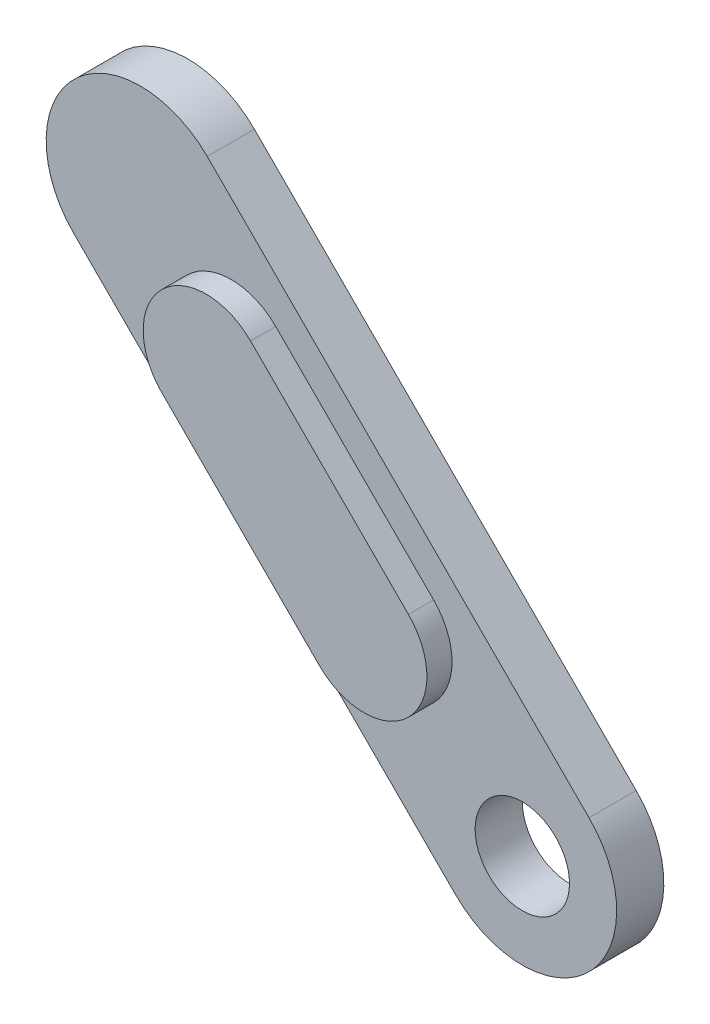
SolidWorks part; units mm, degrees
ref_plane "Front Plane" through (0, 0, 0) normal (0, 0, 1) x (1, 0, 0)
ref_plane "Top Plane" through (0, 0, 0) normal (0, 1, 0) x (1, 0, 0)
ref_plane "Right Plane" through (0, 0, 0) normal (1, 0, 0) x (0, 0, -1)
sketch "Sketch2" plane through (0, 0, 0) normal (0, 0, 1) x (1, 0, 0)
  line L0 (5.5786, 37.7618) -> (-6.5599, 49.9003) construction
  line L1 (7.6999, 39.8831) -> (-4.4386, 52.0216)
  line L2 (3.4572, 35.6405) -> (-8.6812, 47.779)
  arc A0 (3.4572, 35.6405) -> (7.6999, 39.8831) centre (5.5786, 37.7618) ccw
  arc A1 (-4.4386, 52.0216) -> (-8.6812, 47.779) centre (-6.5599, 49.9003) ccw
  dimension "D2" = 3
extrude "Boss-Extrude1" add sketch "Sketch2" along normal blind 1.5
sketch "Sketch3" plane through (0, 0, 1.5) normal (0, 0, 1) x (1, 0, 0)
  line L0 (-3.6751, 47.0155) -> (1.3446, 41.9958) construction
  line L1 (-2.2609, 48.4297) -> (2.7588, 43.41)
  line L2 (-5.0893, 45.6013) -> (-0.0696, 40.5816)
  line L3 (-8.6812, 47.779) -> (3.4572, 35.6405) construction
  arc A0 (-2.2609, 48.4297) -> (-5.0893, 45.6013) centre (-3.6751, 47.0155) ccw
  arc A1 (-0.0696, 40.5816) -> (2.7588, 43.41) centre (1.3446, 41.9958) ccw
  point P2 (-1.1653, 44.5056)
  dimension "D2" = 2
  dimension "D1" = 3
extrude "Boss-Extrude3" add sketch "Sketch3" along normal blind 0.8
sketch "Sketch4" plane through (0, 0, 0) normal (0, 0, -1) x (-1, 0, 0)
  circle A0 centre (-5.5786, 37.7618) radius 1.5
  arc A1 (-7.6999, 39.8831) -> (-3.4572, 35.6405) centre (-5.5786, 37.7618) ccw construction
  dimension "D1" = 3
extrude "Cut-Extrude1" cut sketch "Sketch4" against normal blind 0.8
sketch "Sketch5" plane through (0, 0, 1.5) normal (0, 0, 1) x (1, 0, 0)
  circle A0 centre (-6.5599, 49.9003) radius 1.5
  arc A1 (-4.4386, 52.0216) -> (-8.6812, 47.779) centre (-6.5599, 49.9003) ccw construction
  dimension "D1" = 3
extrude "Cut-Extrude2" cut sketch "Sketch5" against normal blind 13 from offset 0.5 offset against normal yes
sketch "Sketch6" plane through (0, 0, 0) normal (0, 0, -1) x (-1, 0, 0)
  circle A0 centre (-5.5786, 37.7618) radius 1.5 construction
  circle A1 centre (-5.5786, 37.7618) radius 1.5
extrude "Cut-Extrude3" cut sketch "Sketch6" against normal blind 7
